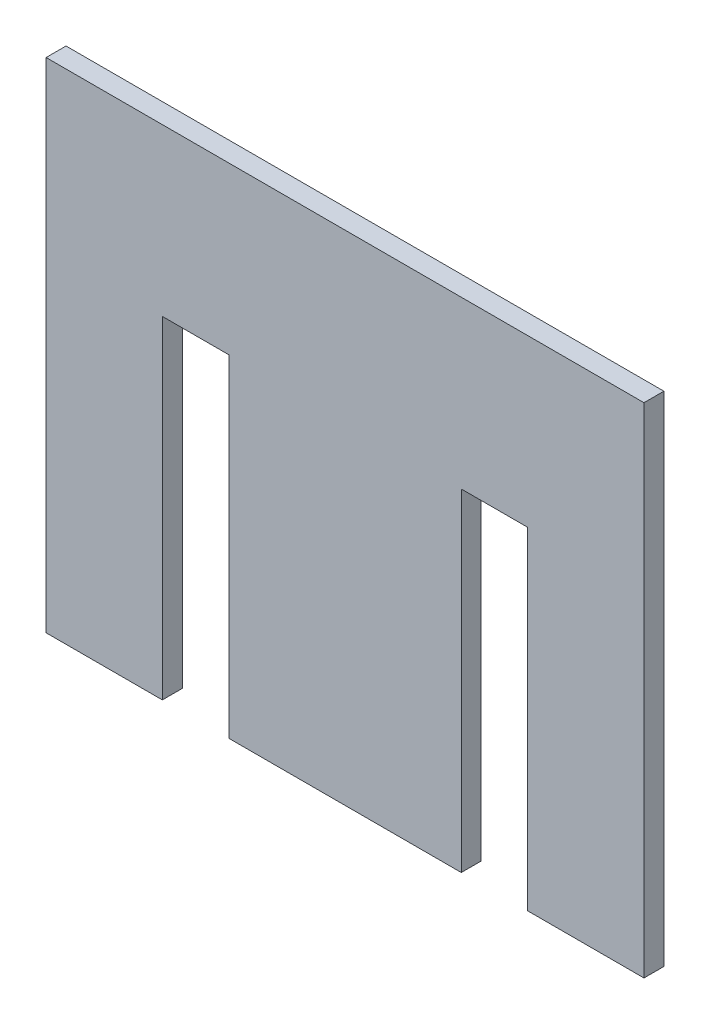
from build123d import *

# Parameters (mm, degrees)
SKETCH_1_W          = 180
SKETCH_1_H          = 150
EXTRUDE_1_DEPTH     = 6
CUT_EXTRUDE_1_REACH = 119.307
SKETCH_2_W          = 20
SKETCH_2_H          = 100


with BuildPart() as part:
    # 草图1 → 凸台-拉伸1 (new body)
    with BuildSketch(Plane.XY):
        Rectangle(SKETCH_1_W, SKETCH_1_H)
    extrude(amount=EXTRUDE_1_DEPTH)

    # 草图2 → 切除-拉伸1 (cut, up to next)
    with BuildSketch(Plane.XY.offset(6), mode=Mode.PRIVATE) as cut_extrude_1_sk1:
        with Locations((-45, -25)):
            Rectangle(SKETCH_2_W, SKETCH_2_H)
    cut_extrude_1_tool1 = extrude(cut_extrude_1_sk1.sketch, amount=-CUT_EXTRUDE_1_REACH, mode=Mode.PRIVATE) & part.part
    cut_extrude_1 = cut_extrude_1_tool1.solids().sort_by_distance((-45, -25, 6))[0]
    add(cut_extrude_1, mode=Mode.SUBTRACT)

    # 镜向1: 切除-拉伸1 across plane
    add(cut_extrude_1.mirror(Plane(origin=(0, 0, 0), x_dir=(0, 0, 1), z_dir=(1, 0, 0))), mode=Mode.SUBTRACT)


solid = part.part
